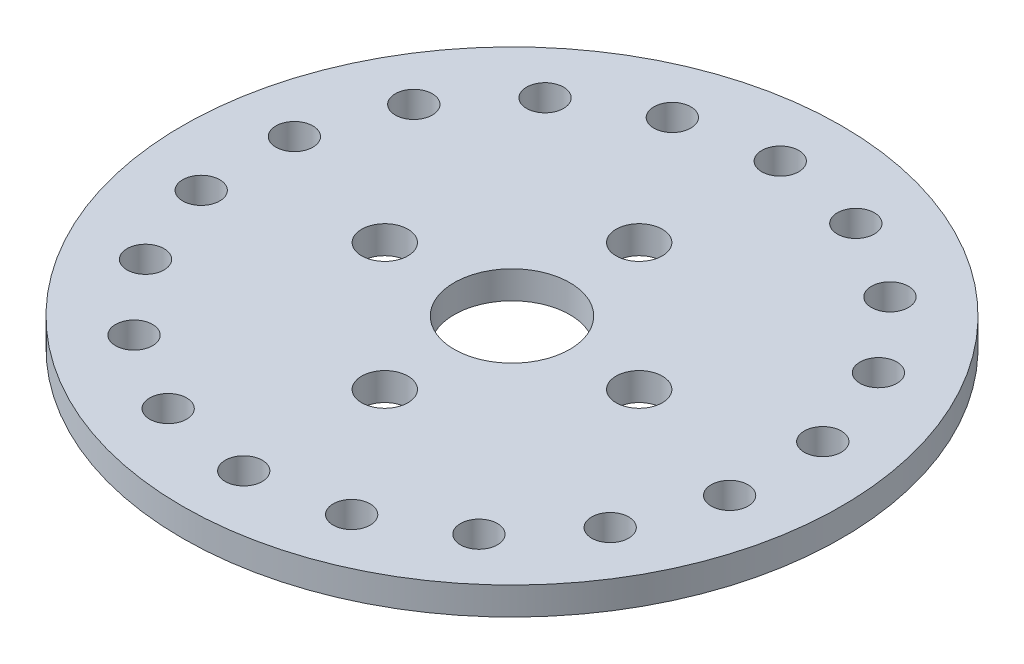
SolidWorks part; units mm, degrees
material "Q235B"
ref_plane "Front Plane" through (0, 0, 0) normal (0, 0, 1) x (1, 0, 0)
ref_plane "Top Plane" through (0, 0, 0) normal (0, 1, 0) x (1, 0, 0)
ref_plane "Right Plane" through (0, 0, 0) normal (1, 0, 0) x (0, 0, -1)
sketch "Sketch1" plane through (0, 0, 0) normal (0, 1, 0) x (1, 0, 0)
  circle A0 centre (0, 0) radius 142.5
  circle A1 centre (0, 0) radius 25
  dimension "D1" = 285
  dimension "D2" = 50
extrude "Boss-Extrude1" add sketch "Sketch1" along normal mid plane 12
hole_wizard "Ø20.0 (20) Diameter Hole1" positions "Sketch2" profile "Sketch3" hole size "Ø20.0" standard "GB" end condition up to next
sketch "Sketch2" plane through (0, 6, 0) normal (0, 1, 0) x (1, 0, 0)
  circle A0 centre (0, 0) radius 55 construction
  point P0 (0, 55)
  point P10 (55, 0)
  point P11 (0, -55)
  point P12 (-55, 0)
  dimension "D1" = 4
  dimension "D2" = 110
sketch "Sketch3" plane through (0, 6, -55) normal (1, 0, 0) x (0, 0, 1)
  line L0 (0, 0) -> (0, 12)
  line L1 (0, 12) -> (10, 12)
  line L2 (10, 12) -> (10, 0)
  line L5 (10, 0) -> (0, 0)
  line L11 (0, -6.35) -> (0, 107.95) construction
  dimension "通孔孔直径" = 20
  dimension "通孔孔深度" = 12
hole_wizard "Ø16.0 (16) Diameter Hole1" positions "Sketch4" profile "Sketch5" hole size "Ø16.0" standard "GB" end condition up to next
sketch "Sketch4" plane through (0, 6, 0) normal (0, 1, 0) x (1, 0, 0)
  circle A1 centre (0, 0) radius 116 construction
  point P0 (0, 116)
  point P7 (39.6743, 109.0043)
  point P8 (74.5634, 88.8612)
  point P9 (100.4589, 58)
  point P10 (114.2377, 20.1432)
  point P11 (114.2377, -20.1432)
  point P12 (100.4589, -58)
  point P13 (74.5634, -88.8612)
  point P14 (39.6743, -109.0043)
  point P15 (0, -116)
  point P16 (-39.6743, -109.0043)
  point P17 (-74.5634, -88.8612)
  point P18 (-100.4589, -58)
  point P19 (-114.2377, -20.1432)
  point P20 (-114.2377, 20.1432)
  point P21 (-100.4589, 58)
  point P22 (-74.5634, 88.8612)
  point P23 (-39.6743, 109.0043)
  dimension "D2" = 232
  dimension "D1" = 18
sketch "Sketch5" plane through (0, 6, -116) normal (1, 0, 0) x (0, 0, 1)
  line L0 (0, 0) -> (0, 12)
  line L1 (0, 12) -> (8, 12)
  line L2 (8, 12) -> (8, 0)
  line L5 (8, 0) -> (0, 0)
  line L11 (0, -6.35) -> (0, 107.95) construction
  dimension "通孔孔直径" = 16
  dimension "通孔孔深度" = 12
